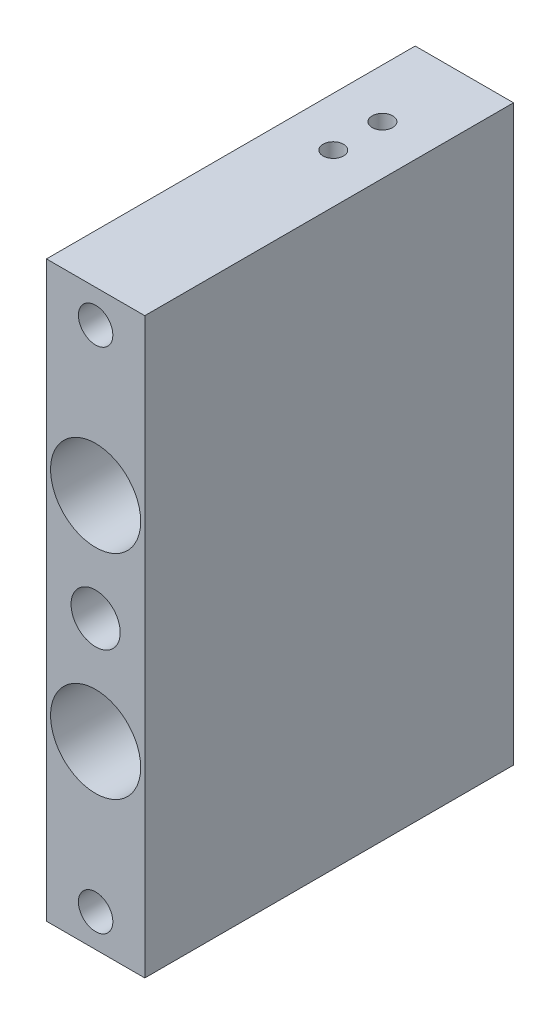
SolidWorks part; units mm, degrees
material "6061铝"
ref_plane "前视基准面" through (0, 0, 0) normal (0, 0, 1) x (1, 0, 0)
ref_plane "上视基准面" through (0, 0, 0) normal (0, 1, 0) x (1, 0, 0)
ref_plane "右视基准面" through (0, 0, 0) normal (1, 0, 0) x (0, 0, -1)
sketch "草图13" plane through (0, 0, 0) normal (0, 0, 1) x (1, 0, 0)
  line L1 (-6, 35) -> (6, 35)
  line L2 (-6, 35) -> (-6, -35)
  line L3 (-6, -35) -> (6, -35)
  line L4 (6, 35) -> (6, -35)
  line L5 (-6, 35) -> (6, -35) construction
  line L6 (-6, -35) -> (6, 35) construction
  point P0 (0, 0)
  dimension "D1" = 12
  dimension "D2" = 70
extrude "凸台-拉伸1" add sketch "草图13" along normal blind 45
hole_wizard "M3 螺纹孔1" positions "草图17" profile "草图18" tap size "M3" standard "GB"
sketch "草图17" plane through (0, 35, 0) normal (0, 1, 0) x (1, 0, 0)
  line L0 (6, 0) -> (-6, 0) construction
  point P0 (0, -10)
  point P6 (0, -16)
  dimension "D1" = 10
  dimension "D2" = 6
sketch "草图18" plane through (0, 35, 10) normal (1, 0, 0) x (0, 0, 1)
  line L0 (0, 0) -> (0, 13.2511)
  line L1 (0, 13.2511) -> (1.25, 12.5)
  line L2 (1.25, 12.5) -> (1.25, 0)
  line L5 (1.25, 0) -> (0, 0)
  line L10 (0, 13.2511) -> (-1.25, 12.5) construction
  line L11 (0, -6.35) -> (0, 107.95) construction
  dimension "螺纹孔钻头直径" = 2.5
  dimension "螺纹孔钻头深度" = 12.5
  dimension "导头角度" = 118
cosmetic thread "孔螺蚊线6" parameters "D1"=10, "D2"=3
cosmetic thread "孔螺蚊线7" parameters "D1"=10, "D2"=3
hole_wizard "M5 螺纹孔1" positions "草图19" profile "草图20" tap size "M5" standard "GB"
sketch "草图19" plane through (0, 0, 45) normal (0, 0, 1) x (1, 0, 0)
  line L0 (0, 31) -> (0, -31) construction
  point P0 (0, 31)
  point P2 (0, -31)
  dimension "D1" = 62
sketch "草图20" plane through (0, 31, 45) normal (1, 0, 0) x (0, -1, 0)
  line L0 (0, 0) -> (0, 20.2618)
  line L1 (0, 20.2618) -> (2.1, 19)
  line L2 (2.1, 19) -> (2.1, 0)
  line L5 (2.1, 0) -> (0, 0)
  line L10 (0, 20.2618) -> (-2.1, 19) construction
  line L11 (0, -6.35) -> (0, 107.95) construction
  dimension "螺纹孔钻头直径" = 4.2
  dimension "螺纹孔钻头深度" = 19
  dimension "导头角度" = 118
cosmetic thread "孔螺蚊线8" parameters "D1"=15, "D2"=5
cosmetic thread "孔螺蚊线9" parameters "D1"=15, "D2"=5
hole_wizard "打孔尺寸(%根据)内六角圆柱头螺钉的类型1" positions "草图21" profile "草图22" counterbore size "M6" standard "GB" end condition through all
sketch "草图21" plane through (0, 0, 45) normal (0, 0, 1) x (1, 0, 0)
  line L0 (0, 13) -> (0, -13) construction
  point P0 (0, 13)
  point P2 (0, -13)
  dimension "D1" = 26
sketch "草图22" plane through (0, 13, 45) normal (1, 0, 0) x (0, -1, 0)
  line L0 (0, 0) -> (0, 45)
  line L1 (0, 45) -> (3.2, 45)
  line L3 (3.2, 45) -> (3.2, 20)
  line L4 (3.2, 20) -> (5.5, 20)
  line L5 (5.5, 20) -> (5.5, 0)
  line L7 (5.5, 0) -> (0, 0)
  line L11 (0, -6.35) -> (0, 107.95) construction
  dimension "通孔孔直径" = 6.4
  dimension "通孔孔深度" = 45
  dimension "柱形沉头孔直径" = 11
  dimension "柱形沉头孔深度" = 20
mirror "镜向1" [suppressed] about plane through (0, 0, 0) normal (0, 1, 0)
hole_wizard "Ø6.0 (6) 直径孔1" positions "草图23" profile "草图25" hole size "Ø6.0" standard "GB"
sketch "草图23" plane through (0, 0, 45) normal (0, 0, 1) x (1, 0, 0)
  point P0 (0, 0)
sketch "草图25" plane through (0, 0, 45) normal (1, 0, 0) x (0, -1, 0)
  line L0 (0, 0) -> (0, 11.8026)
  line L1 (0, 11.8026) -> (3, 10)
  line L2 (3, 10) -> (3, 0)
  line L5 (3, 0) -> (0, 0)
  line L10 (0, 11.8026) -> (-3, 10) construction
  line L11 (0, -6.35) -> (0, 107.95) construction
  dimension "孔直径" = 6
  dimension "孔深度" = 10
  dimension "导头角度" = 118
hole_wizard "Ø6.0 (6) 直径孔2" positions "草图26" profile "草图28" hole size "Ø6.0" standard "GB"
sketch "草图26" plane through (0, 0, 0) normal (0, 0, -1) x (-1, 0, 0)
  line L0 (0, 0) -> (16.8723, 0) construction
  point P0 (0, -22.5)
  point P8 (0, 22.5)
  dimension "D1" = 45
sketch "草图28" plane through (0, -22.5, 0) normal (1, 0, 0) x (0, 1, 0)
  line L0 (0, 0) -> (0, 11.8026)
  line L1 (0, 11.8026) -> (3, 10)
  line L2 (3, 10) -> (3, 0)
  line L5 (3, 0) -> (0, 0)
  line L10 (0, 11.8026) -> (-3, 10) construction
  line L11 (0, -6.35) -> (0, 107.95) construction
  dimension "孔直径" = 6
  dimension "孔深度" = 10
  dimension "导头角度" = 118
